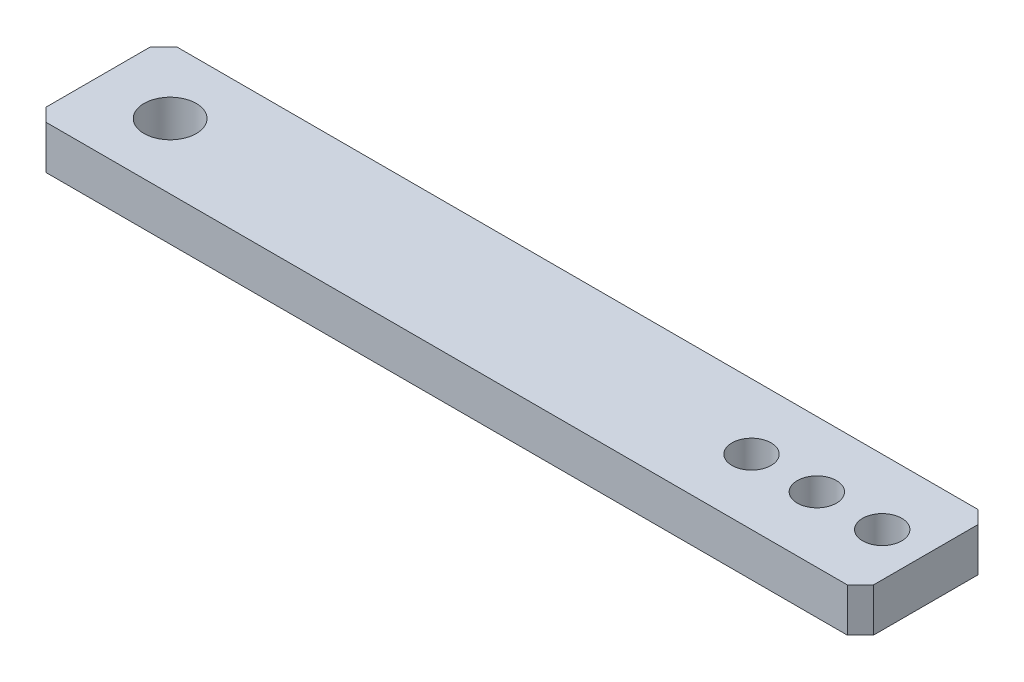
from build123d import *

# Parameters (mm, degrees)
SKETCH1_W                    = 190
SKETCH1_H                    = 30
BOSS_EXTRUDE1_DEPTH          = 10
CHAMFER1_SIZE                = 3
F_9_0_9_DIAMETER_HOLE1_D     = 9
F_9_0_9_DIAMETER_HOLE1_DEPTH = 19.75
F_9_0_9_DIAMETER_HOLE1_TIP   = 2.703872786
F_9_0_9_DIAMETER_HOLE2_D     = 12
F_9_0_9_DIAMETER_HOLE2_DEPTH = 19.75
F_9_0_9_DIAMETER_HOLE2_TIP   = 3.605163714


with BuildPart() as part:
    # Sketch1 → Boss-Extrude1 (new body)
    with BuildSketch(Plane(origin=(0, 0, 0), x_dir=(1, 0, 0), z_dir=(0, 1, 0))):
        Rectangle(SKETCH1_W, SKETCH1_H)
    extrude(amount=BOSS_EXTRUDE1_DEPTH)

    # Chamfer1
    chamfer1_edges = [part.edges().sort_by_distance(p)[0] for p in [
        (95, 5, 15),
        (-95, 5, 15),
        (-95, 5, -15),
        (95, 5, -15),
    ]]
    chamfer(chamfer1_edges, length=CHAMFER1_SIZE)

    # Ø9.0 (9) Diameter Hole1
    with Locations(Plane(origin=(0, 10, 0), x_dir=(1, 0, 0), z_dir=(0, 1, 0))):
        with Locations((85, 0), (70, 0), (55, 0)):
            Hole(F_9_0_9_DIAMETER_HOLE1_D / 2, depth=F_9_0_9_DIAMETER_HOLE1_DEPTH)
            with Locations((0, 0, -(F_9_0_9_DIAMETER_HOLE1_DEPTH + F_9_0_9_DIAMETER_HOLE1_TIP / 2))):  # 118° drill point
                Cone(0, F_9_0_9_DIAMETER_HOLE1_D / 2, F_9_0_9_DIAMETER_HOLE1_TIP, mode=Mode.SUBTRACT)

    # Ø9.0 (9) Diameter Hole2
    with Locations(Plane(origin=(0, 0, 0), x_dir=(-1, 0, 0), z_dir=(0, -1, 0))):
        with Locations((78.492424049, 0)):
            Hole(F_9_0_9_DIAMETER_HOLE2_D / 2, depth=F_9_0_9_DIAMETER_HOLE2_DEPTH)
            with Locations((0, 0, -(F_9_0_9_DIAMETER_HOLE2_DEPTH + F_9_0_9_DIAMETER_HOLE2_TIP / 2))):  # 118° drill point
                Cone(0, F_9_0_9_DIAMETER_HOLE2_D / 2, F_9_0_9_DIAMETER_HOLE2_TIP, mode=Mode.SUBTRACT)


solid = part.part
